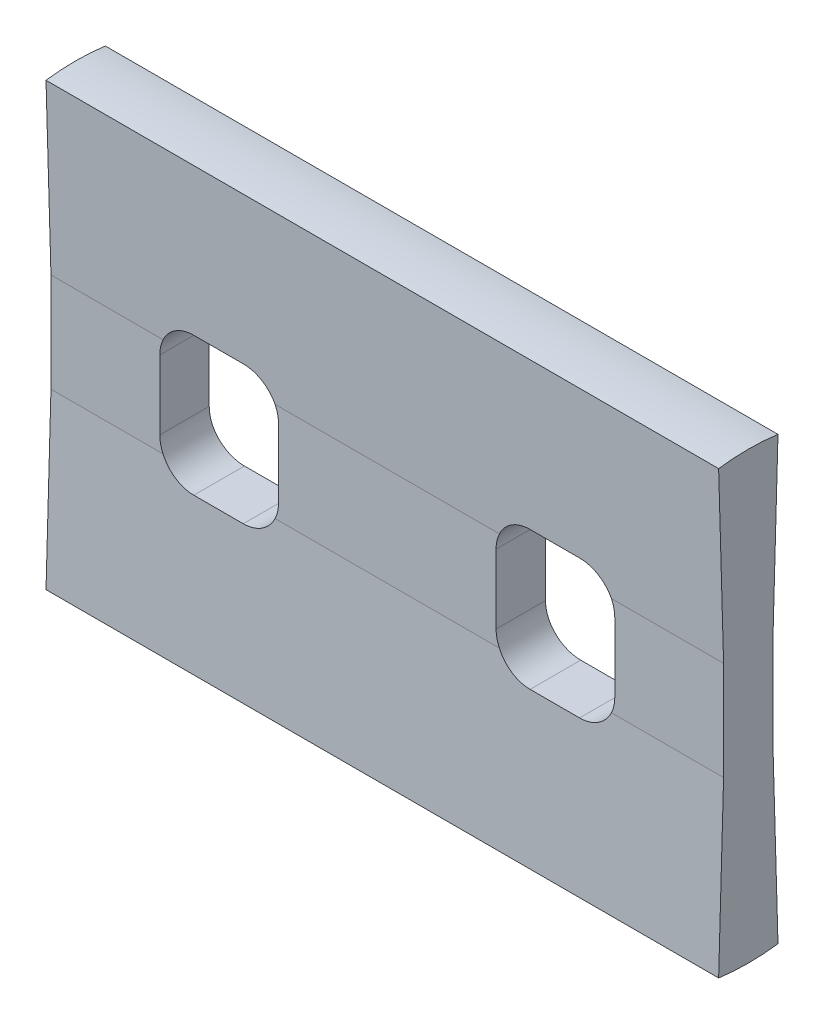
SolidWorks part; units mm, degrees
material "灰铸铁 HT150 "
ref_plane "Front Plane" through (0, 0, 0) normal (0, 0, 1) x (1, 0, 0)
ref_plane "Top Plane" through (0, 0, 0) normal (0, 1, 0) x (1, 0, 0)
ref_plane "Right Plane" through (0, 0, 0) normal (1, 0, 0) x (0, 0, -1)
sketch "Sketch1" plane through (0, 0, 0) normal (1, 0, 0) x (0, 0, -1)
  line L0 (0, -177.4306) -> (0, 177.4306) construction
  line L1 (111.1111, 0) -> (-111.1111, 0) construction
  line L2 (25, -50) -> (25, 50)
  line L3 (25, 50) -> (30, 222.991)
  line L4 (-25, 50) -> (-30, 222.991)
  line L5 (-25, -50) -> (-25, 50)
  line L6 (-25, -50) -> (-30, -222.991)
  line L7 (25, -50) -> (30, -222.991)
  arc A0 (-30, -222.991) -> (30, -222.991) centre (0, 0) ccw
  arc A1 (30, 222.991) -> (-30, 222.991) centre (0, 0) ccw
  point P4 (0, 0)
  point P8 (0, 0)
  point P15 (-25, 0)
  point P18 (25, 0)
  dimension "D4" = 450
  dimension "D1" = 50
  dimension "D2" = 60
  dimension "D3" = 50
  dimension "D5" = 60
extrude "Boss-Extrude1" add sketch "Sketch1" along normal mid plane 680
sketch "Sketch2" plane through (0, 0, 0) normal (0, 0, 1) x (1, 0, 0)
  line L0 (0, -304.4972) -> (0, 304.4972) construction
  line L1 (388.6122, 0) -> (-388.6122, 0) construction
  line L3 (-145, -70) -> (-195, -70)
  line L4 (-110, -35) -> (-110, 35)
  line L5 (-145, 70) -> (-195, 70)
  line L6 (-230, -35) -> (-230, 35)
  line L7 (-110, -70) -> (-230, 70) construction
  line L8 (-110, 70) -> (-230, -70) construction
  arc A0 (-145, -70) -> (-110, -35) centre (-145, -35) ccw
  arc A1 (-195, -70) -> (-230, -35) centre (-195, -35) cw
  arc A2 (-230, 35) -> (-195, 70) centre (-195, 35) cw
  arc A3 (-110, 35) -> (-145, 70) centre (-145, 35) ccw
  point P0 (-170, 0)
  point P4 (0, 0)
  point P8 (0, 0)
  dimension "D4" = 35
  dimension "D1" = 120
  dimension "D2" = 140
  dimension "D3" = 170
extrude "Cut-Extrude1" cut sketch "Sketch2" against normal through all both and the other way through all
mirror "Mirror1" about plane through (0, 0, 0) normal (1, 0, 0) of "Cut-Extrude1"
